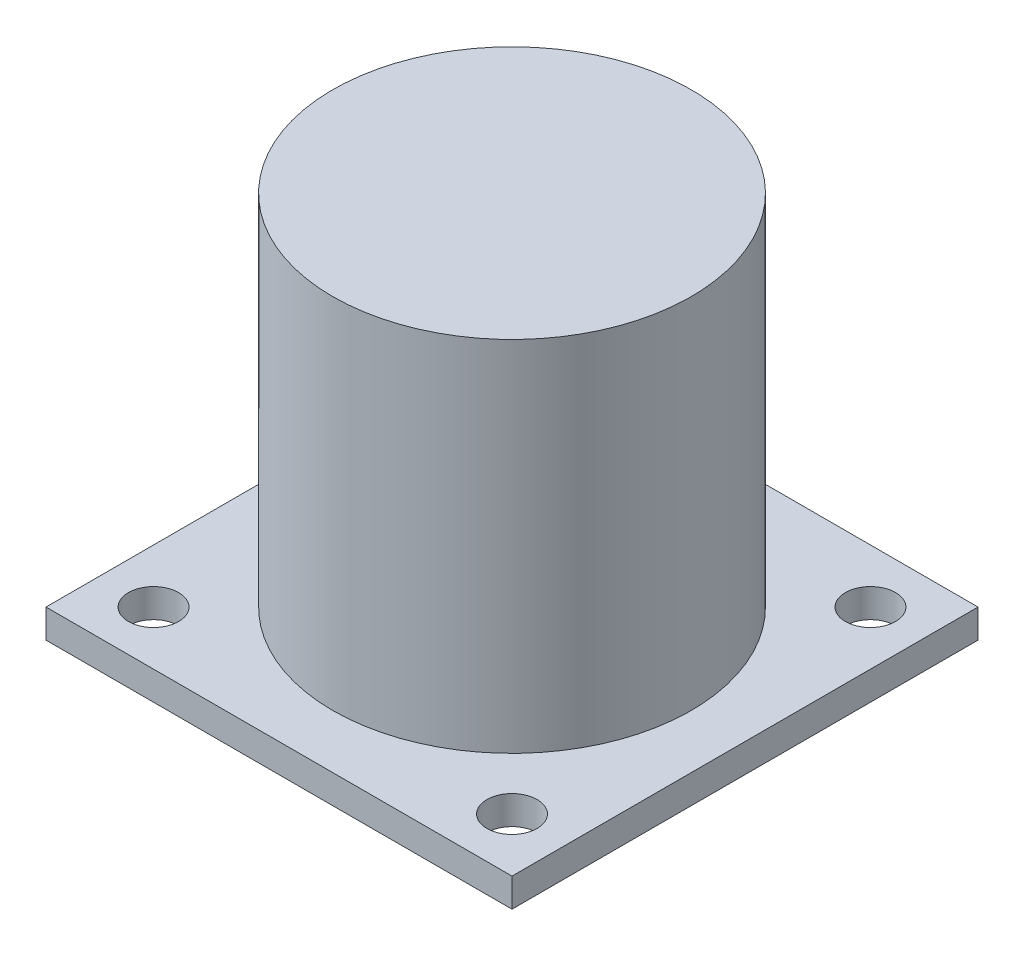
SolidWorks part; units mm, degrees
material "Q235B"
ref_plane "Front Plane" through (0, 0, 0) normal (0, 0, 1) x (1, 0, 0)
ref_plane "Top Plane" through (0, 0, 0) normal (0, 1, 0) x (1, 0, 0)
ref_plane "Right Plane" through (0, 0, 0) normal (1, 0, 0) x (0, 0, -1)
sketch "Sketch1" plane through (0, 0, 0) normal (0, 1, 0) x (1, 0, 0)
  line L1 (65, -65) -> (-65, -65)
  line L2 (65, -65) -> (65, 65)
  line L3 (65, 65) -> (-65, 65)
  line L4 (-65, -65) -> (-65, 65)
  line L5 (65, -65) -> (-65, 65) construction
  line L6 (65, 65) -> (-65, -65) construction
  point P0 (0, 0)
  dimension "D1" = 130
extrude "Boss-Extrude1" add sketch "Sketch1" along normal blind 8
sketch "Sketch2" plane through (0, 8, 0) normal (0, 1, 0) x (1, 0, 0)
  circle A0 centre (0, 0) radius 50
  dimension "D1" = 100
extrude "Boss-Extrude2" add sketch "Sketch2" along normal blind 100
hole_wizard "Ø14.0 (14) Diameter Hole1" positions "Sketch3" profile "Sketch4" hole size "Ø14.0" standard "GB"
sketch "Sketch3" plane through (0, 8, 0) normal (0, 1, 0) x (1, 0, 0)
  line L0 (0, 65) -> (0, 0) construction
  line L1 (65, 65) -> (-65, 65) construction
  line L2 (0, 0) -> (-65, 0) construction
  line L3 (-65, 65) -> (-65, -65) construction
  point P0 (-50, 50)
  point P12 (50, 50)
  point P13 (50, -50)
  point P14 (-50, -50)
  dimension "D1" = 100
  dimension "D2" = 100
sketch "Sketch4" plane through (-50, 8, -50) normal (1, 0, 0) x (0, 0, 1)
  line L0 (0, 0) -> (0, 26.206)
  line L1 (0, 26.206) -> (7, 22)
  line L2 (7, 22) -> (7, 0)
  line L5 (7, 0) -> (0, 0)
  line L10 (0, 26.206) -> (-7, 22) construction
  line L11 (0, -6.35) -> (0, 107.95) construction
  dimension "孔直径" = 14
  dimension "孔深度" = 22
  dimension "导头角度" = 118
